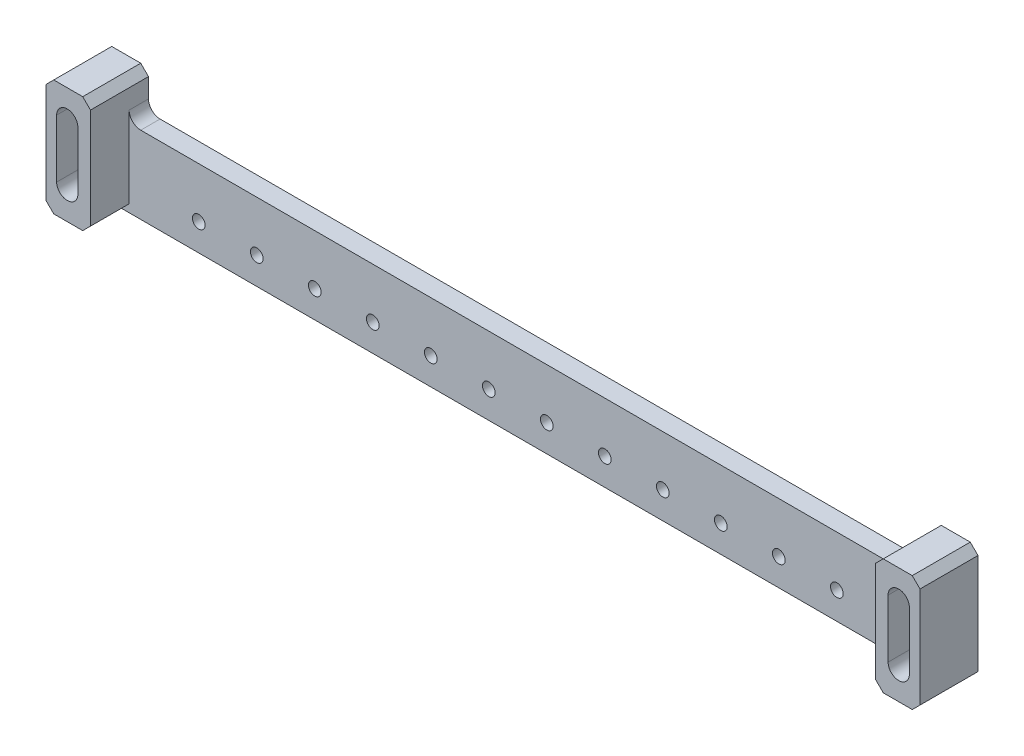
SolidWorks part; units mm, degrees
ref_plane "前视基准面" through (0, 0, 0) normal (0, 0, 1) x (1, 0, 0)
ref_plane "上视基准面" through (0, 0, 0) normal (0, 1, 0) x (1, 0, 0)
ref_plane "右视基准面" through (0, 0, 0) normal (1, 0, 0) x (0, 0, -1)
sketch "草图1" plane through (0, 0, 0) normal (0, 0, 1) x (1, 0, 0)
  line L1 (-113, -15) -> (113, -15)
  line L2 (-113, -15) -> (-113, 15)
  line L3 (-113, 15) -> (113, 15)
  line L4 (113, -15) -> (113, 15)
  line L5 (-113, -15) -> (113, 15) construction
  line L6 (-113, 15) -> (113, -15) construction
  point P0 (0, 0)
  dimension "D1" = 226
  dimension "D2" = 30
extrude "凸台-拉伸1" add sketch "草图1" along normal blind 15
sketch "草图2" plane through (0, 0, 15) normal (0, 0, 1) x (1, 0, 0)
  line L0 (113, 15) -> (-113, 15) construction
  line L1 (-101.5, -15) -> (101.5, -15)
  line L2 (-101.5, -15) -> (-101.5, 15)
  line L3 (-101.5, 15) -> (101.5, 15)
  line L4 (101.5, -15) -> (101.5, 15)
  line L5 (-101.5, -15) -> (101.5, 15) construction
  line L6 (-101.5, 15) -> (101.5, -15) construction
  line L7 (-113, 15) -> (-113, -15) construction
  point P0 (0, 0)
  dimension "D1" = 11.5
extrude "切除-拉伸1" cut sketch "草图2" against normal blind 10
sketch "草图3" plane through (0, 0, 5) normal (0, 0, 1) x (1, 0, 0)
  line L0 (101.5, -15) -> (101.5, 15) construction
  line L1 (-101.5, 15) -> (101.5, 15)
  line L2 (-101.5, 15) -> (-101.5, 5)
  line L3 (-101.5, 5) -> (101.5, 5)
  line L4 (101.5, 15) -> (101.5, 5)
  dimension "D1" = 10
extrude "切除-拉伸2" cut sketch "草图3" against normal through all
sketch "草图4" plane through (0, 0, 0) normal (0, 0, -1) x (-1, 0, 0)
  line L0 (107.5, -7.5) -> (107.5, 7.5) construction
  line L1 (104.75, -7.5) -> (104.75, 7.5)
  line L2 (110.25, -7.5) -> (110.25, 7.5)
  line L3 (-107.5, -7.5) -> (-107.5, 7.5) construction
  line L4 (-110.25, -7.5) -> (-110.25, 7.5)
  line L5 (-104.75, -7.5) -> (-104.75, 7.5)
  line L6 (113, 15) -> (113, -15) construction
  line L7 (0, 0) -> (0, -15) construction
  line L8 (113, -15) -> (-113, -15) construction
  line L9 (101.5, 15) -> (113, 15) construction
  arc A0 (104.75, -7.5) -> (110.25, -7.5) centre (107.5, -7.5) ccw
  arc A1 (110.25, 7.5) -> (104.75, 7.5) centre (107.5, 7.5) ccw
  arc A2 (-110.25, -7.5) -> (-104.75, -7.5) centre (-107.5, -7.5) ccw
  arc A3 (-104.75, 7.5) -> (-110.25, 7.5) centre (-107.5, 7.5) ccw
  point P2 (107.5, 0)
  point P7 (-107.5, 0)
  point P21 (0, 0)
  dimension "D1" = 15
  dimension "D2" = 5.5
  dimension "D3" = 5.5
  dimension "D4" = 15
extrude "切除-拉伸3" cut sketch "草图4" against normal through all
sketch "草图5" plane through (0, 0, 0) normal (0, 0, -1) x (-1, 0, 0)
  line L0 (107.5, -7.5) -> (107.5, 7.5) construction
  line L1 (102.5, -7.5) -> (102.5, 7.5)
  line L2 (112.5, -7.5) -> (112.5, 7.5)
  line L3 (-107.5, -7.5) -> (-107.5, 7.5) construction
  line L4 (-112.5, -7.5) -> (-112.5, 7.5)
  line L5 (-102.5, -7.5) -> (-102.5, 7.5)
  arc A0 (102.5, -7.5) -> (112.5, -7.5) centre (107.5, -7.5) ccw
  arc A1 (112.5, 7.5) -> (102.5, 7.5) centre (107.5, 7.5) ccw
  arc A2 (-112.5, -7.5) -> (-102.5, -7.5) centre (-107.5, -7.5) ccw
  arc A3 (-102.5, 7.5) -> (-112.5, 7.5) centre (-107.5, 7.5) ccw
  point P4 (107.5, 0)
  point P9 (-107.5, 0)
  dimension "D1" = 10
extrude "切除-拉伸4" cut sketch "草图5" against normal blind 6
hole_wizard "M4 螺纹孔1" positions "草图6" profile "草图7" tap size "M4" standard "GB" end condition through all
sketch "草图6" plane through (0, 0, 0) normal (0, 0, -1) x (-1, 0, 0)
  line L0 (113, -15) -> (-113, -15) construction
  line L1 (-113, -15) -> (-113, 15) construction
  point P0 (-81.5, -8)
  dimension "D1" = 7
  dimension "D2" = 31.5
sketch "草图7" plane through (81.5, -8, 0) normal (1, 0, 0) x (0, 1, 0)
  line L0 (0, 0) -> (0, 15)
  line L1 (0, 15) -> (1.65, 15)
  line L2 (1.65, 15) -> (1.65, 0)
  line L5 (1.65, 0) -> (0, 0)
  line L11 (0, -6.35) -> (0, 107.95) construction
  dimension "通孔螺纹孔钻头直径" = 3.3
  dimension "通孔螺纹孔钻头深度" = 15
cosmetic thread "孔螺蚊线1" parameters "D2"=4
pattern_linear "阵列(线性)1" count 12 spacing 15 along (-1, 0, 0) of "M4 螺纹孔1"
chamfer "倒角1" distance 2 angle 45 8 edges at (113, 15, 7.5) (101.5, 15, 7.5) (113, -15, 7.5) (101.5, -15, 10) (-113, -15, 7.5) (-101.5, -15, 10) (-101.5, 15, 7.5) (-113, 15, 7.5)
fillet "圆角1" radius 3 2 edges at (101.5, 5, 2.5) (-101.5, 5, 2.5)
